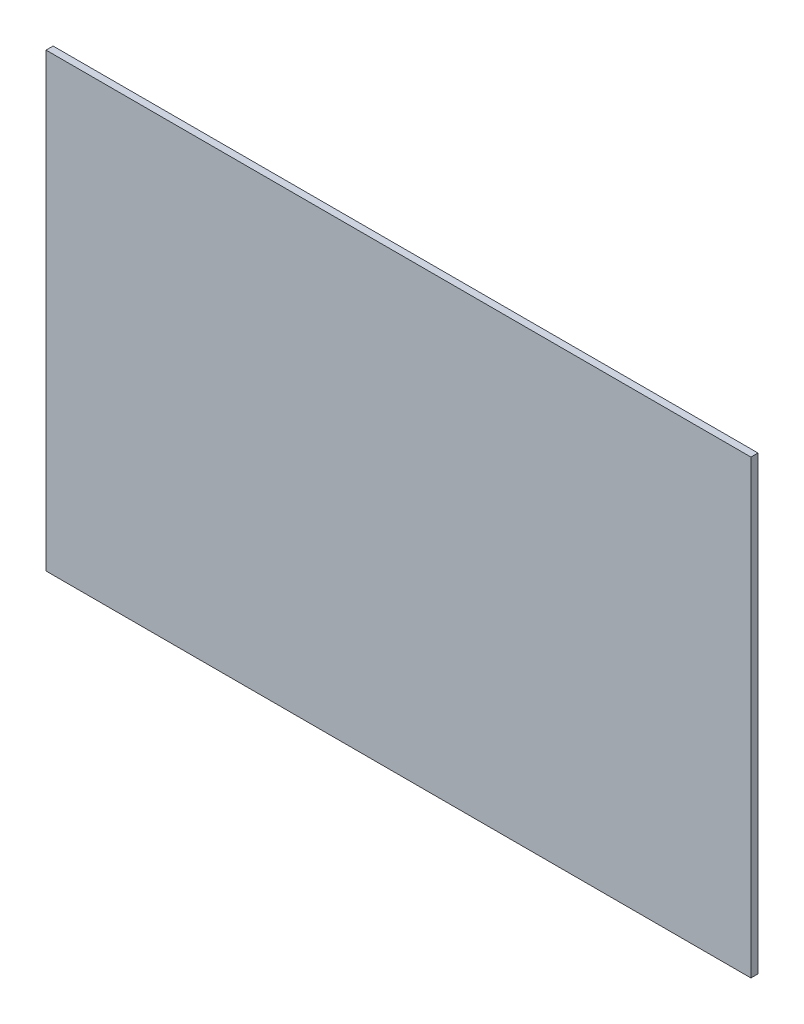
from build123d import *

# Parameters (mm, degrees)
SKETCH1_W           = 500
SKETCH1_H           = 320
BOSS_EXTRUDE1_DEPTH = 5


with BuildPart() as part:
    # Sketch1 → Boss-Extrude1 (new body)
    with BuildSketch(Plane.XY):
        with Locations((250, 160)):
            Rectangle(SKETCH1_W, SKETCH1_H)
    extrude(amount=BOSS_EXTRUDE1_DEPTH)


solid = part.part
